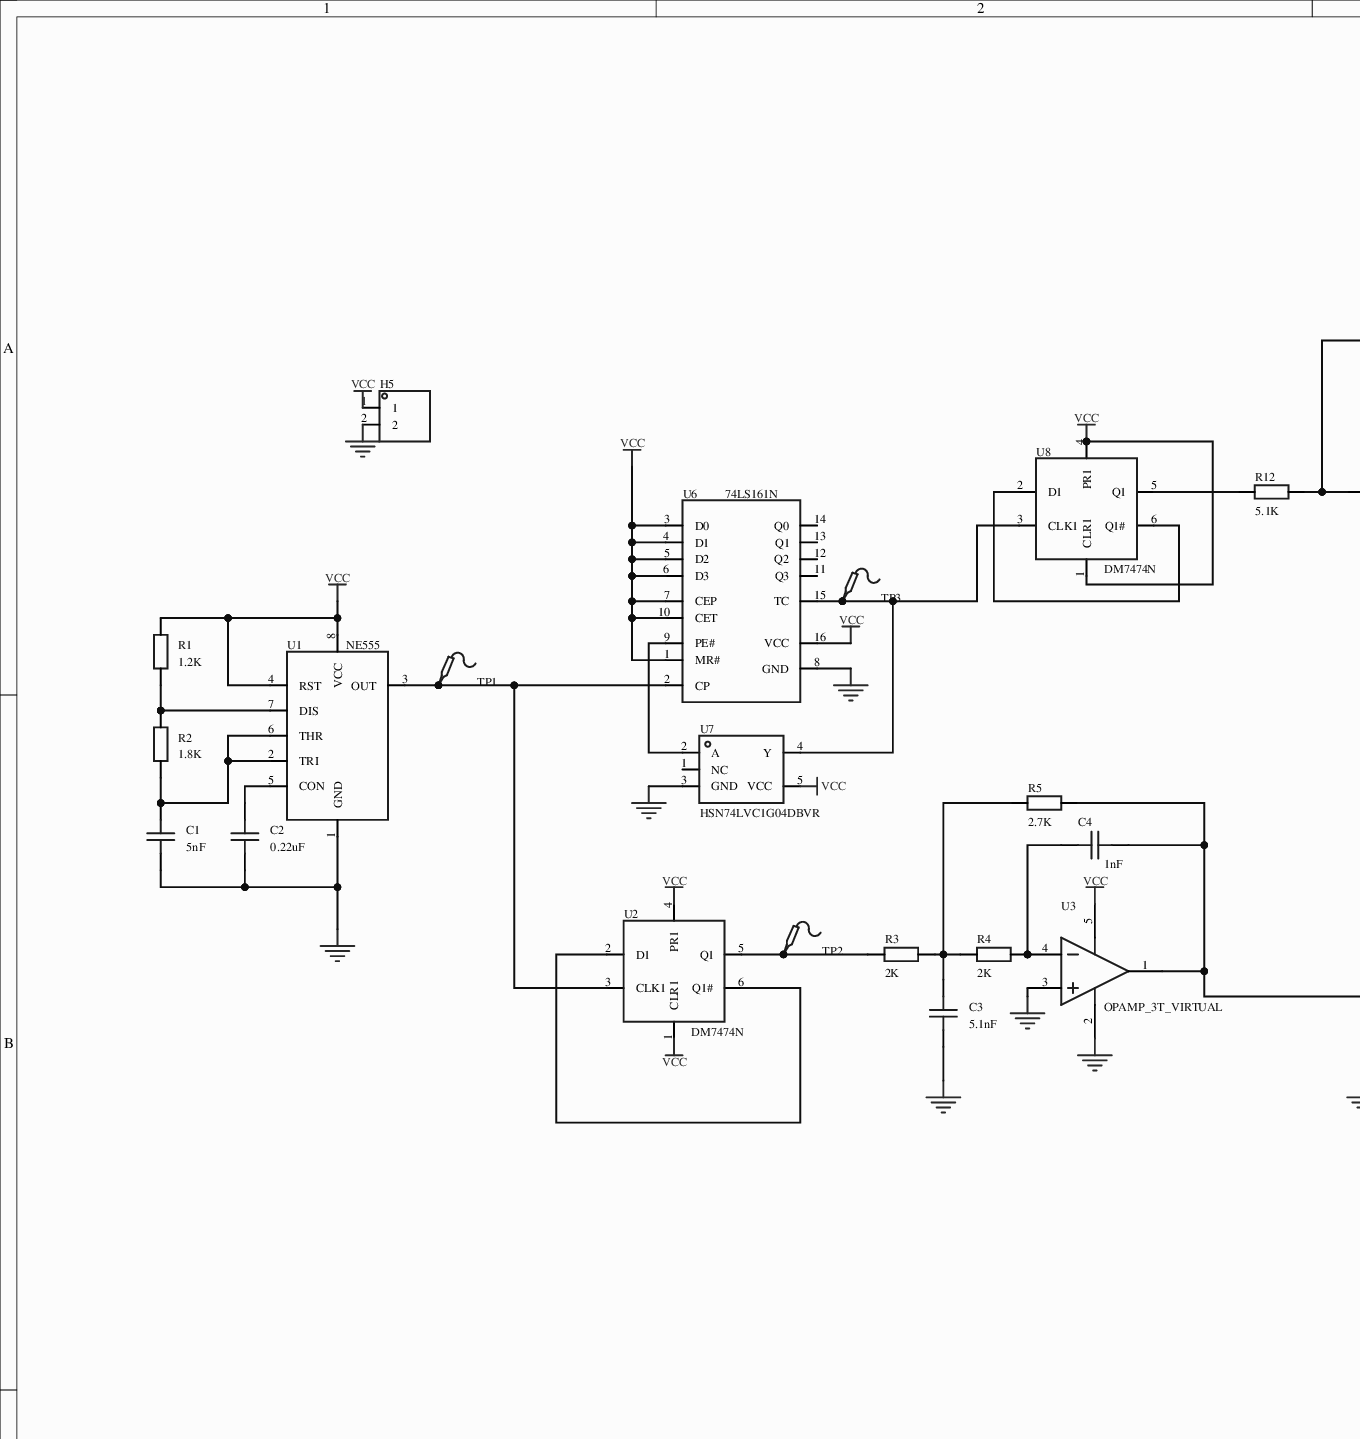
[diagram p0: MISC51901-3.schdoc, top left]
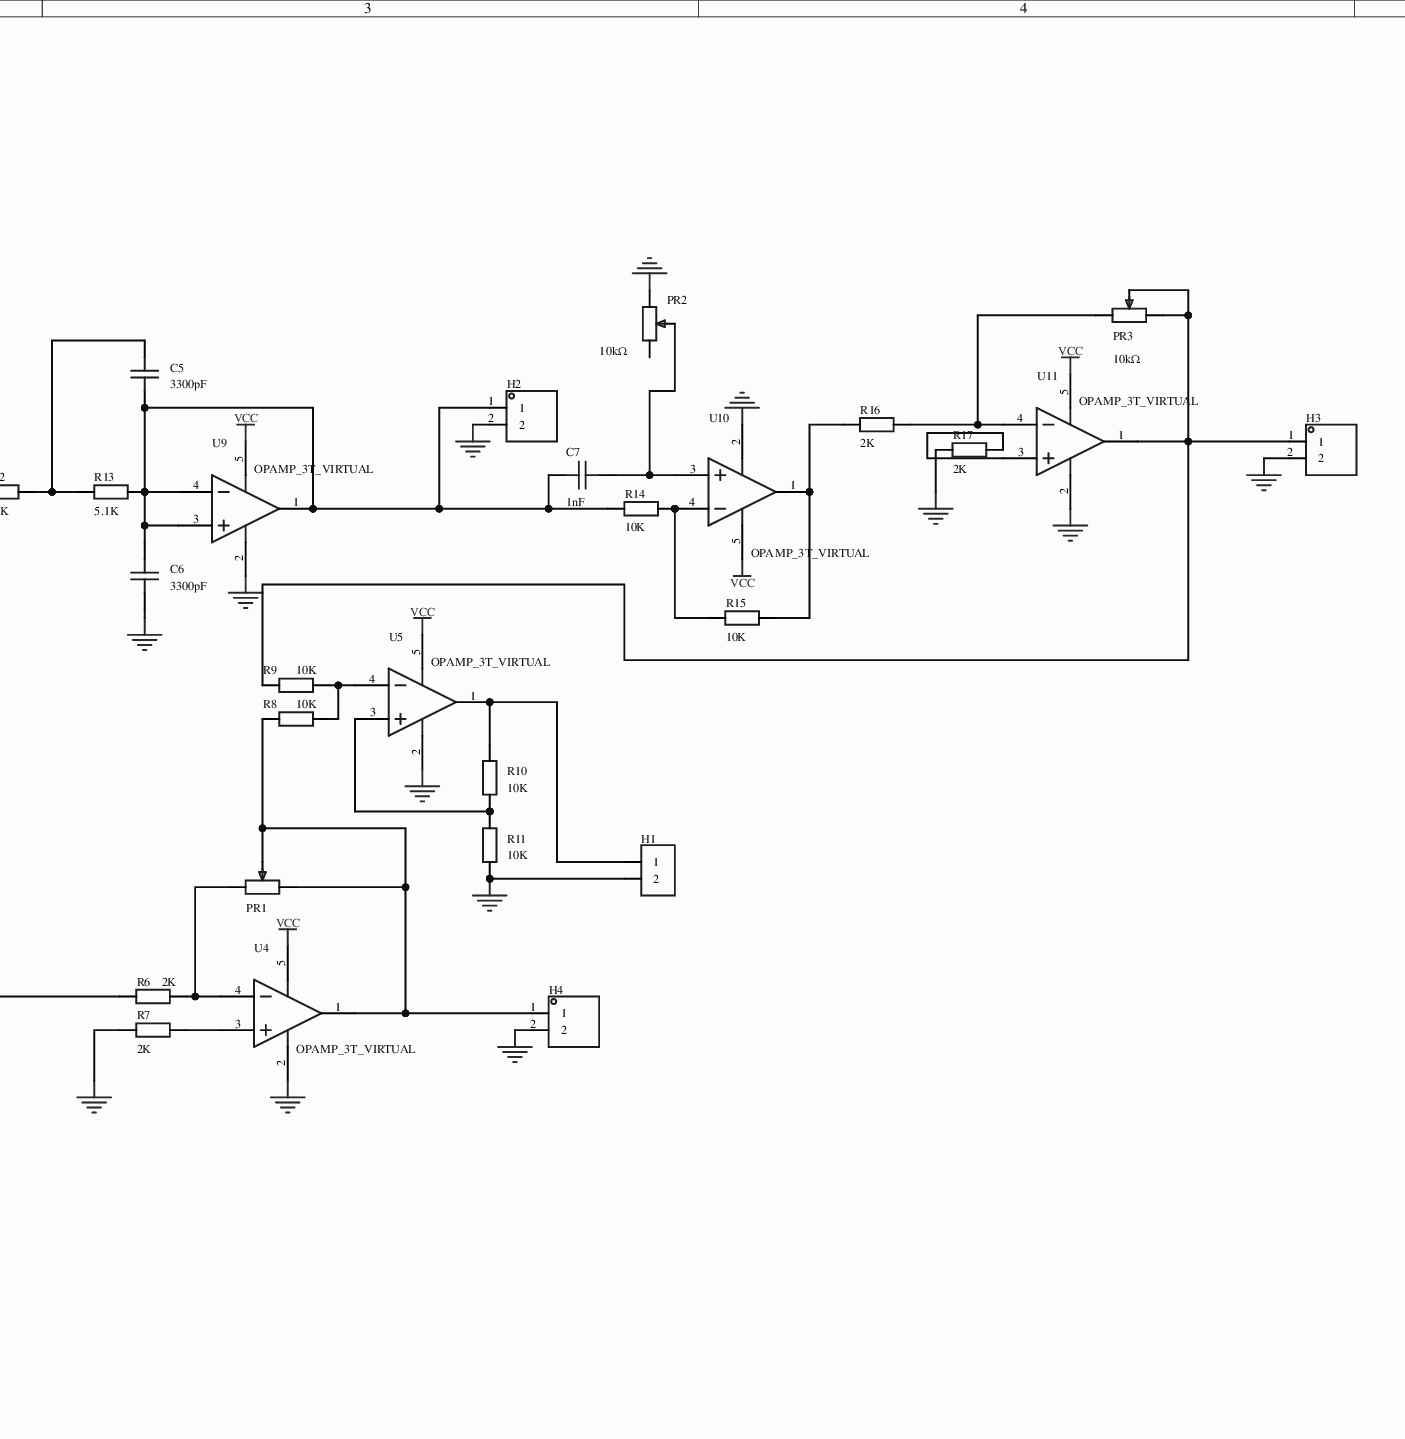
[diagram p1: MISC51901-3.schdoc, top middle]
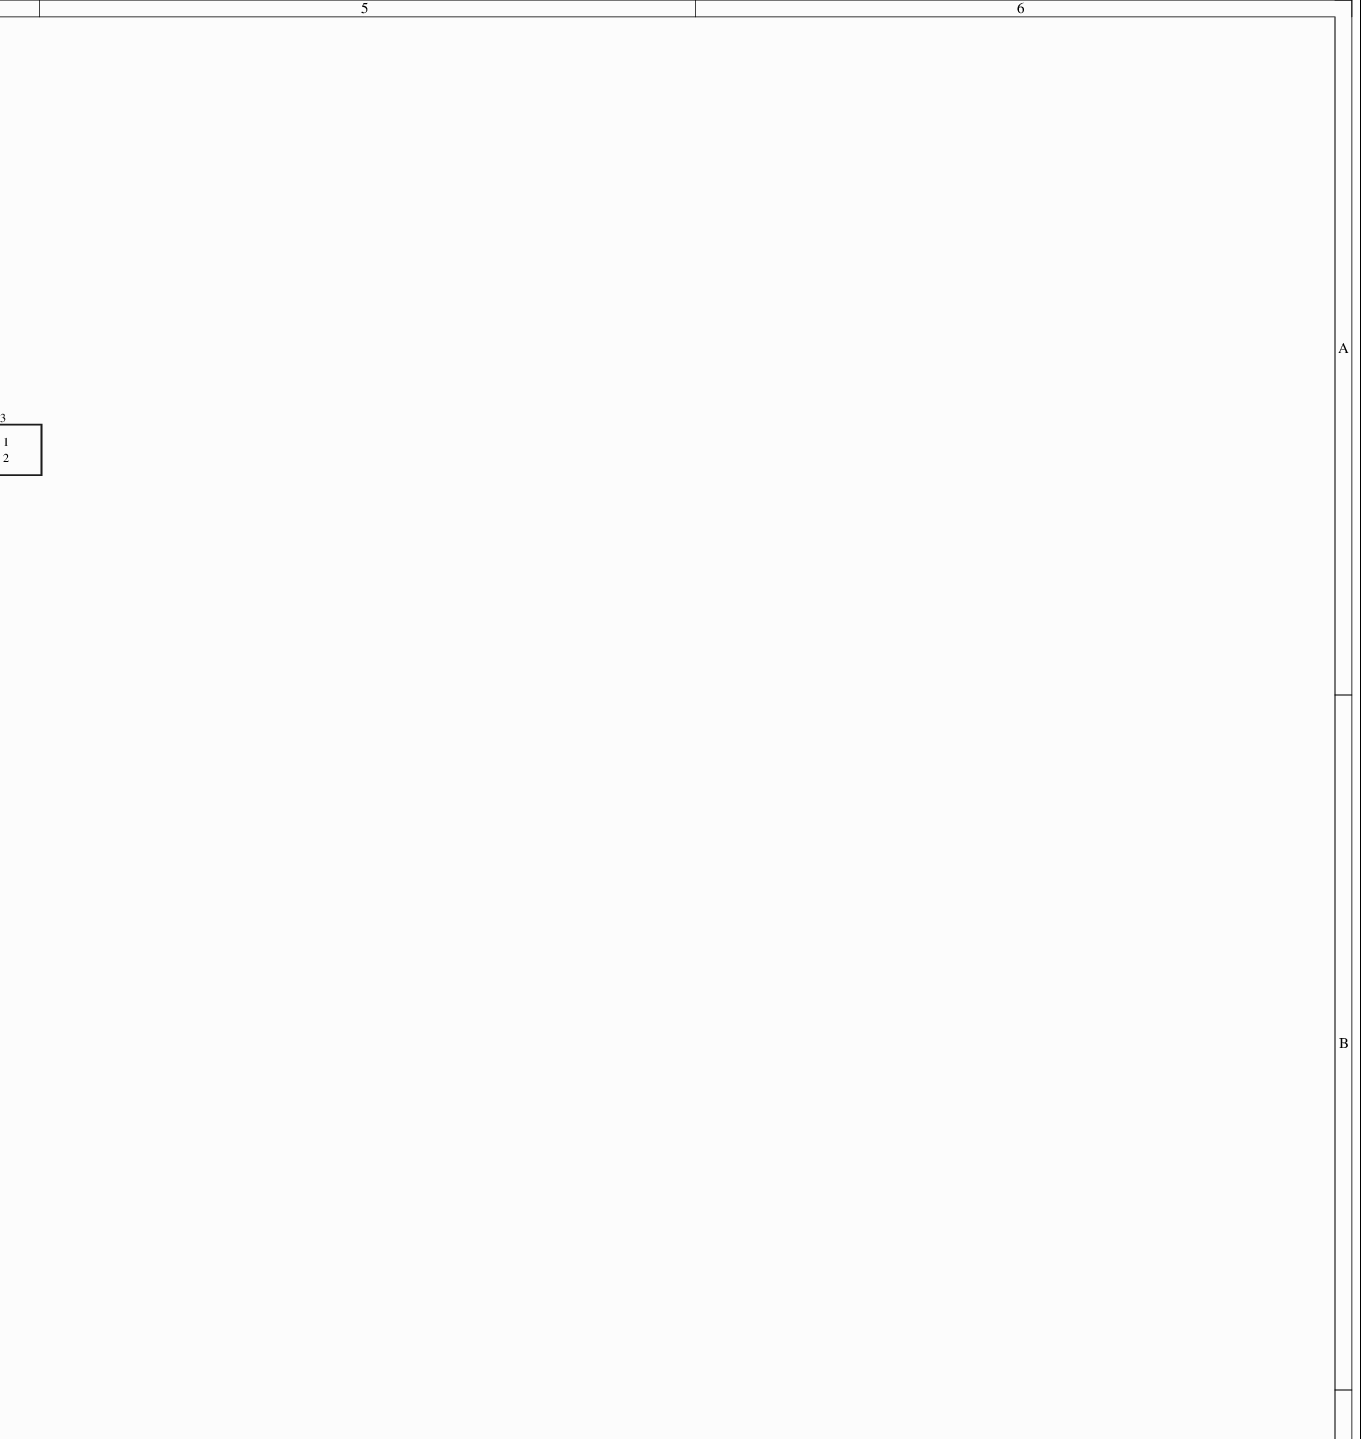
[diagram p2: MISC51901-3.schdoc, top right]
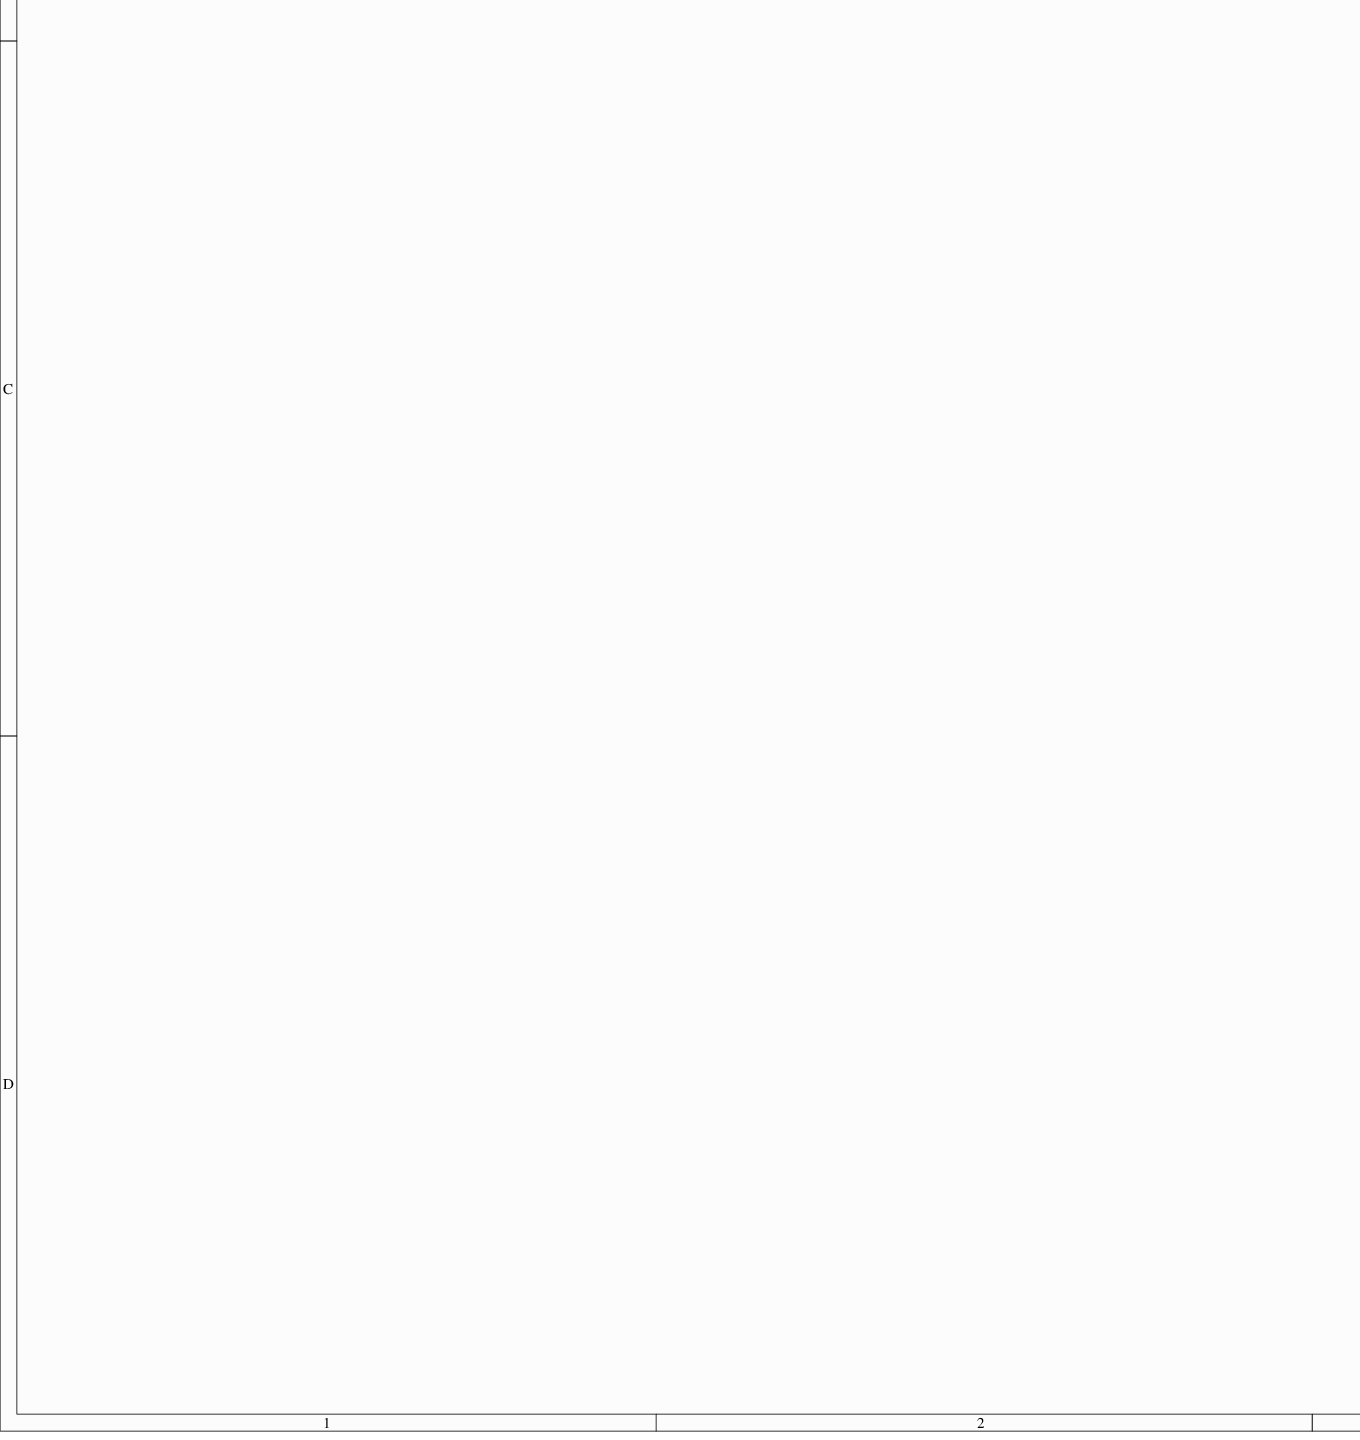
[diagram p3: MISC51901-3.schdoc, bottom left]
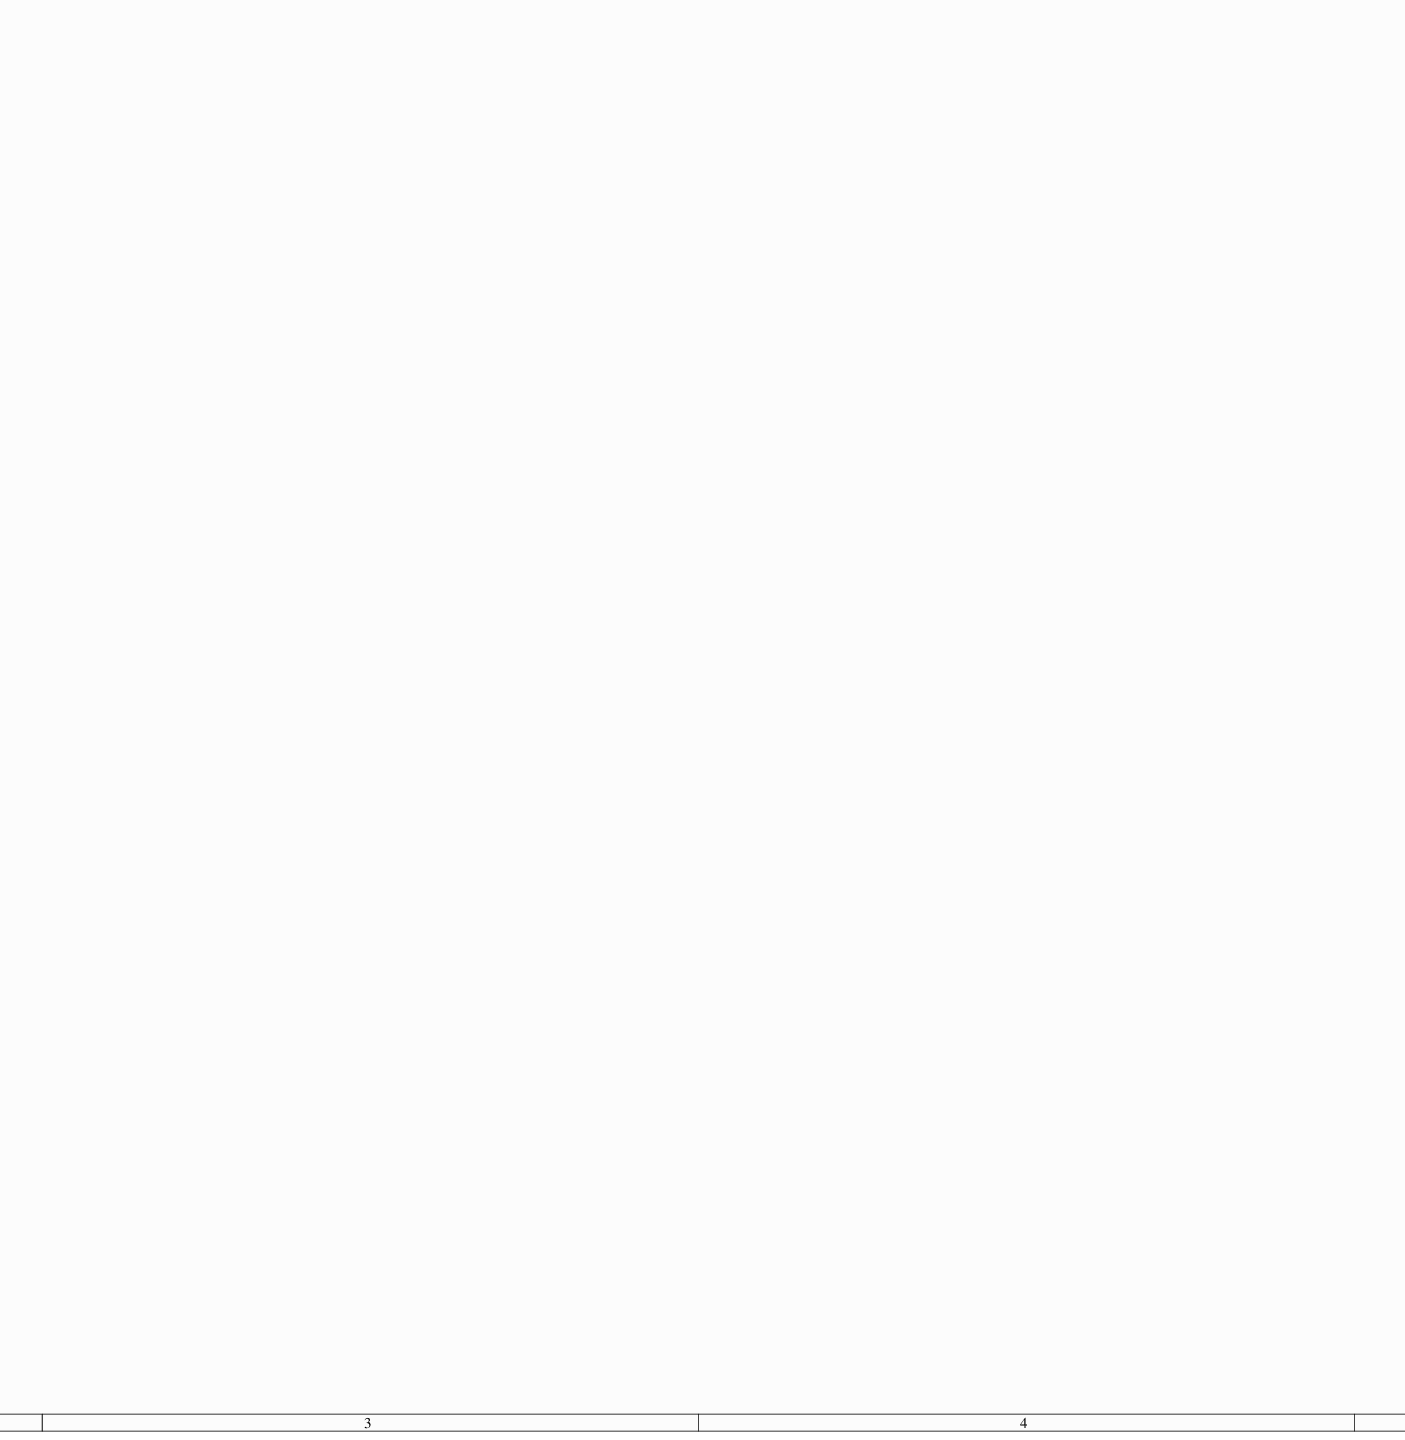
[diagram p4: MISC51901-3.schdoc, bottom middle]
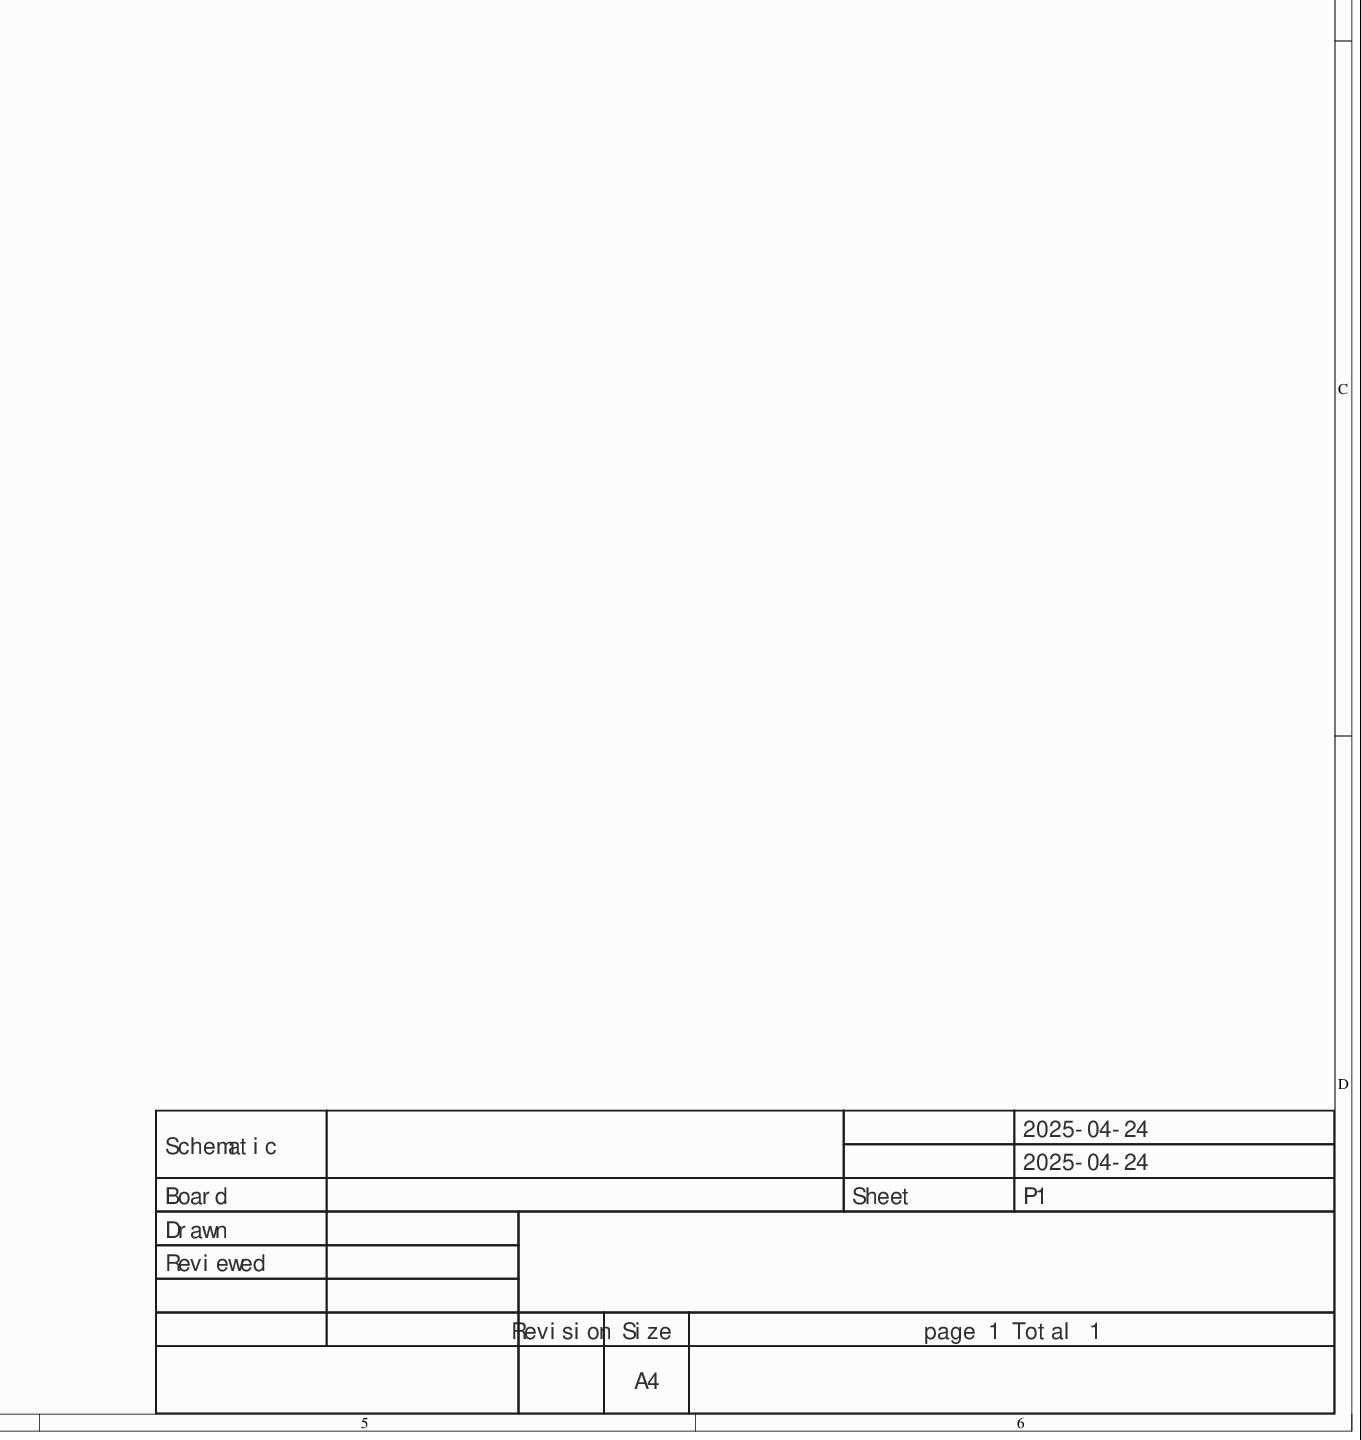
[diagram p5: MISC51901-3.schdoc, bottom right]
# Altium project MISC51901-2.PrjPcb
1 sheet, 46 parts. Net scope: global (net labels, ports and power ports of the same name join across sheets).
Board file: MISC51901.pcbdoc

## Sheet MISC51901-3.schdoc
size 594 x 419 mm; Version: V1.0; @Project Name: MISC51901; @Page Count: 1; @Update Date: 2025-04-24; @Create Date: 2025-04-24; @Schematic Name: MISC51901; @Page No: 1; @Create Time: 19:51:46; @Update Time: 21:09:39; @Board Name: MISC51901

### Parts
C1  5nF  [C0603]
C2  0.22uF  [C0603]
C3  5.1nF  [C0603]
C4  1nF  [C0603]
C5  3300pF  [C0603]
C6  3300pF  [C0603]
C7  1nF  [C0603]
H1  (no value)  [HDR-TH_2P-P2.54-V-F]
H2  (no value)  [HDR-TH_2P-P2.54-V-M-1]
H3  (no value)  [HDR-TH_2P-P2.54-V-M-1]
H4  (no value)  [HDR-TH_2P-P2.54-V-M-1]
H5  (no value)  [HDR-TH_2P-P2.54-V-M-1]
PR1  10kΩ  [R_3296]  (value not drawn)
PR2  10kΩ  [R_3296]
PR3  10kΩ  [R_3296]
R1  1.2K  [R0603]
R2  1.8K  [R0603]
R3  2K  [R0603]
R4  2K  [R0603]
R5  2.7K  [R0603]
R6  2K  [R0603]
R7  2K  [R0603]
R8  10K  [R0603]
R9  10K  [R0603]
R10  10K  [R0603]
R11  10K  [R0603]
R12  5.1K  [R0603]
R13  5.1K  [R0603]
R14  10K  [R0603]
R15  10K  [R0603]
R16  2K  [R0603]
R17  2K  [R0603]
TP1  (no value)  [Test-Point-0.5mm]
TP2  (no value)  [Test-Point-0.5mm]
TP3  (no value)  [Test-Point-0.5mm]
U1  NE555  [PDIP-8_L9.6-W6.4-P2.54-LS7.9-BL-1]
U2  DM7474N  [PDIP-14_L19.5-W6.7-P2.54-LS7.9-BL]
U3  OPAMP_3T_VIRTUAL  [SOT-23-5_L3.0-W1.7-P0.95-LS2.8-BR]
U4  OPAMP_3T_VIRTUAL  [SOT-23-5_L3.0-W1.7-P0.95-LS2.8-BR]
U5  OPAMP_3T_VIRTUAL  [SOT-23-5_L3.0-W1.7-P0.95-LS2.8-BR]
U6  74LS161N  [PDIP-16_L19.3-W6.4-P2.54-LS7.94-BL]
U7  HSN74LVC1G04DBVR  [SOT-23-5_L2.9-W1.6-P0.95-LS2.9-BL]
U8  DM7474N  [PDIP-14_L19.5-W6.7-P2.54-LS7.9-BL]
U9  OPAMP_3T_VIRTUAL  [SOT-23-5_L3.0-W1.7-P0.95-LS2.8-BR]
U10  OPAMP_3T_VIRTUAL  [SOT-23-5_L3.0-W1.7-P0.95-LS2.8-BR]
U11  OPAMP_3T_VIRTUAL  [SOT-23-5_L3.0-W1.7-P0.95-LS2.8-BR]

### Nets
GND: C1.1 C2.1 C3.1 C6.1 H1.2 H2.2 H3.2 H4.2 H5.2 PR2.3 R7.1 R11.1 R17.1 U1.1(GND) U3.2(V-) U3.3(IN+) U4.2(V-) U5.2(V-) U6.8(GND) U7.3(GND) U9.2(V-) U10.2(V-) U11.2(V-)
VCC: H5.1 R1.2 U1.4(RST) U1.8(VCC) U2.1(CLR1) U2.4(PR1) U3.5(V+) U4.5(V+) U5.5(V+) U6.1(MR#) U6.3(D0) U6.4(D1) U6.5(D2) U6.6(D3) U6.7(CEP) U6.10(CET) U6.16(VCC) U7.5(VCC) U8.1(CLR1) U8.4(PR1) U9.5(V+) U10.5(V+) U11.5(V+)
NetC1_2: C1.2 R2.1 U1.2(TRI) U1.6(THR)
NetC2_2: C2.2 U1.5(CON)
NetC3_2: C3.2 R3.2 R4.1 R5.1
NetC4_1: C4.1 R4.2 U3.4(IN-)
NetC4_2: C4.2 R5.2 R6.1 U3.1(OUT)
NetC5_1: C5.1 C6.2 C7.2 H2.1 R13.2 R14.1 U9.1(OUT) U9.3(IN+) U9.4(IN-)
NetC5_2: C5.2 R12.2 R13.1
NetC7_1: C7.1 PR2.2 U10.3(IN+)
NetH1_1: H1.1 R10.2 U5.1(OUT)
NetH3_1: H3.1 PR3.1 PR3.2 R9.1 U11.1(OUT)
NetH4_1: H4.1 PR1.1 PR1.2 R8.1 U4.1(OUT)
NetPR1_3: PR1.3 R6.2 U4.4(IN-)
NetPR3_3: PR3.3 R16.2 U11.4(IN-)
NetR1_1: R1.1 R2.2 U1.7(DIS)
NetR3_1: R3.1 TP2.1 U2.5(Q1)
NetR7_2: R7.2 U4.3(IN+)
NetR8_2: R8.2 R9.2 U5.4(IN-)
NetR10_1: R10.1 R11.2 U5.3(IN+)
NetR12_1: R12.1 U8.5(Q1)
NetR14_2: R14.2 R15.1 U10.4(IN-)
NetR15_2: R15.2 R16.1 U10.1(OUT)
NetR17_2: R17.2 U11.3(IN+)
NetTP1_1: TP1.1 U1.3(OUT) U2.3(CLK1) U6.2(CP)
NetTP3_1: TP3.1 U6.15(TC) U7.4(Y) U8.3(CLK1)
NetU2_2: U2.2(D1) U2.6(Q1#)
NetU6_9: U6.9(PE#) U7.2(A)
NetU8_2: U8.2(D1) U8.6(Q1#)

Not connected (* = marked no-connect by the designer): PR2 1; U6 11(Q3) 12(Q2) 13(Q1) 14(Q0); U7 1(NC)*

### Notes on the sheet
- 2025-04-24
- Schematic
- Board
- Sheet
- P1
- Drawn
- Reviewed
- Revision
- Size
- A4
- page 1 Total 1

### Library data of the parts
C1-C7 = CAP_0603: ConvertToPcb: yes; SymbolName: CapAcitance; ModelId: ac125912035d415993ca9572d50418b1; ModelName: C0603_L1.6-W0.8-H0.8; ModelTransform: 62.992,31.496,0,0,0,0,0,0,0; Device: CAP_0603; AddInBom: yes; Supplier Footprint: 0603; FootprintName: C0603
  C1: Value: 5nF
  C2: Value: 0.22uF
  C3: Value: 5.1nF
  C4 C7: Value: 1nF
  C5 C6: Value: 3300pF
H1 = HDR-F_2.54_1x2P: Symbol: Header-Female-2.54_1x2; ConvertToPcb: yes; ModelId: a9450ef445564560a104363b9aacde4e; ModelName: HDR-TH_2P-P2.54-F-LI-1X2P; ModelTransform: 215.7476,98.425,0,0,0,0,0,0,-129.921; Device: HDR-F_2.54_1x2P; AddInBom: yes; SupplierPart: C49661; Supplier Footprint: 插件; FootprintName: HDR-TH_2P-P2.54-V-F
H2-H5 = HDR-M_2.54_1x2P: Symbol: 210S-1*2P L=11.6MMGold-plated black; ConvertToPcb: yes; ModelId: 79b2e9f2d70a4d68a1b7098f27c6d4c5; ModelName: HDR-M-2.54_1x2; ModelTransform: 200,100,0,0,0,0,0,0,-118.11; Device: HDR-M_2.54_1x2P; AddInBom: yes; SupplierPart: C124375; Supplier Footprint: 插件; FootprintName: HDR-TH_2P-P2.54-V-M-1
PR1-PR3 = R_3296: ConvertToPcb: yes; ModelId: b182808559bb43bda9e7de64b64134cb; ModelName: 3296W; ModelTransform: 373.98,188.96,590.49,180,0,0,0,0,-140; Device: R_3296; AddInBom: yes; Supplier Footprint: 直插; SymbolName: R_3296; FootprintName: R_3296; Value: 10kΩ
R1-R17 = Res_0603: ConvertToPcb: yes; SymbolName: Resistor; ModelId: fc143cca1e79419f9cd78b61e9279f08; ModelTransform: 31.8897,63.7794,0,90,0,0,0,0,0; Device: Res_0603; AddInBom: yes; Supplier Footprint: 0603; FootprintName: R0603; ModelName: R0603
  R1: Value: 1.2K
  R2: Value: 1.8K
  R3 R4 R6 R7 R16 R17: Value: 2K
  R5: Value: 2.7K
  R8-R11 R14 R15: Value: 10K
  R12 R13: Value: 5.1K
TP1-TP3 = Test-Point: Test Point; AddInBom: yes; Device: Test-Point; ConvertToPcb: yes; SymbolName: Test-Point; FootprintName: Test-Point-0.5mm
U1 = NE555PE4: NE555 single-precision timer; Manufacturer: TI(德州仪器); AddInBom: yes; ModelId: 1b8eaf096e7944deafe216467068c10e; ModelTransform: 377.952,318.897,0,0,0,0,0,0,-118.11; Manufacturer Part: NE555; Symbol: NE555PE4; Device: NE555PE4; LCSC Part Name: NE555PE4; SupplierPart: C2859604; Supplier Footprint: PDIP-8; JLCPCB Part Class: Extended; Supplier: LCSC; ConvertToPcb: yes; FootprintName: PDIP-8_L9.6-W6.4-P2.54-LS7.9-BL-1; ModelName: PDIP-8_L9.6-W6.4-P2.54-LS7.9-BL-1
U2 U8 = DM7474N: Type: D-type; supply voltage: 4.75V~5.25V; clock frequency: 15MHz; elements: 2; bits per element: 1; max propagation delay: 40ns@5V,15pF; quiescent current (Iq): 30mA;; Manufacturer: TI(德州仪器); AddInBom: yes; Trigger Type: Rising edge; Function: Set and reset; Number of Elements: 2; Number of Bits per Element: 1; Output Type: Complementary; Sink Current: 16mA; Source Current: 400uA; ModelId: 54e4a14e1c964e4d8957b52ed5aa85d9; ModelTransform: 767.715,311.023,0,0,0,0,0,0,-129.921; Symbol: DM7474N; Device: DM7474N; LCSC Part Name: DM7474N; SupplierPart: C3827260; ManufacturerPart: DM7474N; Supplier Footprint: PDIP-14; JLCPCB Part Class: Extended; Datasheet: https://atta.szlcsc.com/upload/public/pdf/source/20230915/F50CE702BE5FBF5B3D20FC95F075EAF5.pdf; Supplier: LCSC; ConvertToPcb: yes; Supply Voltage: 4.75V~5.25V; Clock Frequency: 15MHz; Maximum Propagation Delay: 40ns@5V,15pF; Series: 7400 series; Quiescent Current (Iq): 30mA; Operating Temperature: 0℃~+70℃; FootprintName: PDIP-14_L19.5-W6.7-P2.54-LS7.9-BL; ModelName: PDIP-14_L19.5-W6.7-P2.54-LS7.9-BL
U3-U5 U9-U11 = OPA376AIDBVOPAMPSOT23-5: AddInBom: yes; ModelId: 0a2a1b8f50944f73965918ad6e5fe167; ModelName: SOT-23-5_L2.9-W1.6-H1.1-LS2.8-P0.95; ModelTransform: 114.173,109.636,0,180,0,0,0,0,0; Symbol: OPA376AIDBVOPAMPSOT23-5; Manufacturer Part: OPAMP_3T_VIRTUAL; Device: OPA376AIDBVOPAMPSOT23-5; LCSC Part Name: OPA376AIDBVOPAMPSOT23-5; SupplierPart: C9900089405; Supplier Footprint: SOT-23-5; Supplier: LCSC; ConvertToPcb: yes; FootprintName: SOT-23-5_L3.0-W1.7-P0.95-LS2.8-BR
U6 = SN74LS161N(LX): Operating voltage: 2V~6V; elements: 1; trigger edge: rising edge; count rate: 27MHz;; Manufacturer: LX(灵星芯微); AddInBom: yes; Logic Type: Divide by 2; Direction: Up counter; Number of Elements: 1; Reset: Asynchronous; Timing: Synchronous; ModelId: 96ff5d01b3074dd183bcbc4cd00a63de; ModelTransform: 759.841,322.44,0,0,0,0,0,0,-137.795; Manufacturer Part: 74LS161N; Symbol: SN74LS161N(LX); Device: SN74LS161N(LX); LCSC Part Name: SN74LS161N(LX); SupplierPart: C22449622; Supplier Footprint: DIP-16; JLCPCB Part Class: Extended; Datasheet: https://atta.szlcsc.com/upload/public/pdf/source/20240603/93FAE93C61248A77FCA8A2A231F511F6.pdf; Supplier: LCSC; ConvertToPcb: yes; Voltage - Supply: 2V~6V; Trigger Type: Rising edge; Count Rate: 27MHz; Operating Temperature: -40℃~+125℃; FootprintName: PDIP-16_L19.3-W6.4-P2.54-LS7.94-BL; ModelName: PDIP-16_L19.3-W6.4-P2.54-LS7.94-BL
U7 = HSN74LVC1G04DBVR: Logic type: inverter; channels: 1; operating voltage: 1.65V~5.5V; quiescent current (Iq): 10uA;; Manufacturer: HXY MOSFET(华轩阳电子); AddInBom: yes; ModelId: f208335ea6894ff1b04bfab971ca745a; ModelTransform: 114.173,114.173,0,0,0,0,0,-0.003,0; Number of Channels: 1; Symbol: HSN74LVC1G04DBVR; Device: HSN74LVC1G04DBVR; LCSC Part Name: 非门 通道数:1 电源:1.65V~5.5V 静态电流:10uA; SupplierPart: C22396398; ManufacturerPart: HSN74LVC1G04DBVR; Supplier Footprint: SOT-23-5L; Datasheet: https://atta.szlcsc.com/upload/public/pdf/source/20240509/AD7545420B9880DDD4BED8C2101454EC.pdf; Supplier: LCSC; ConvertToPcb: yes; FootprintName: SOT-23-5_L2.9-W1.6-P0.95-LS2.9-BL; ModelName: SOT-23-5_L2.9-W1.6-P0.95-LS2.9-BL; Logic Type: Inverter; Voltage - Supply: 1.65V~5.5V; Quiescent Current: 10uA; Current - Output Low(IOL): -; Current - Output High(IOH): -; Input Logic Level - High: -; Input Logic Level - Low: -; Output Logic Level - High: -